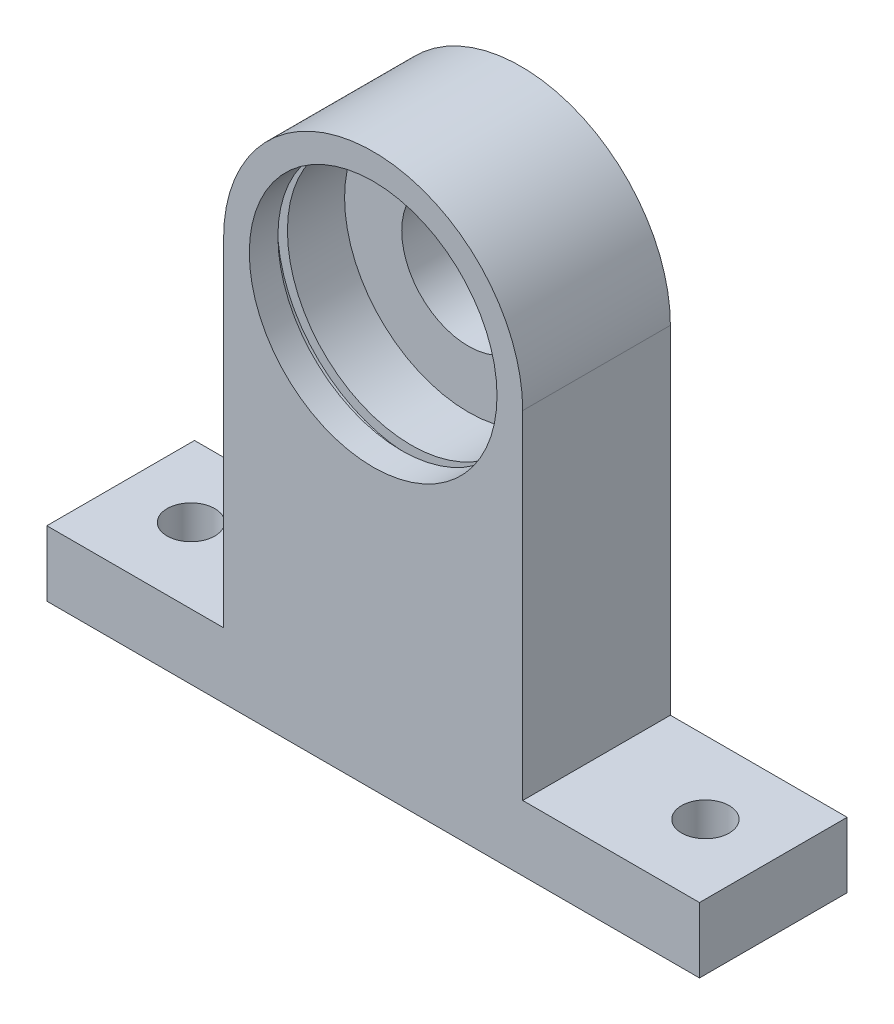
from build123d import *

# Parameters (mm, degrees)
SKETCH1_R           = 31.396947085
SKETCH1_R_2         = 12.5
BOSS_EXTRUDE1_DEPTH = 31
SKETCH2_R           = 5
CUT_EXTRUDE1_DEPTH  = 31
SKETCH3_R           = 14
CUT_EXTRUDE2_DEPTH  = 114.19357359
SKETCH5_R           = 26
CUT_EXTRUDE4_DEPTH  = 20
SKETCH6_R           = 28.1
CUT_EXTRUDE5_DEPTH  = 2


with BuildPart() as part:
    # Sketch1 → Boss-Extrude1 (new body)
    # profile 1 of 2: a face of its own
    with BuildSketch(Plane.XY):
        Circle(SKETCH1_R)
        with Locations(Location((0, 0, 0), (0, 0, 180))):
            Circle(SKETCH1_R_2, mode=Mode.SUBTRACT)
    # profile 2 of 2: a face of its own
    with BuildSketch(Plane.XY):
        with BuildLine():
            ThreePointArc((31.396947085, 0), (0, -31.396947085), (-31.396947085, 0))
            Line((-31.396947085, 0), (-31.396947085, -70.888581066))
            Line((-31.396947085, -70.888581066), (-68.506708087, -70.888581066))
            Line((-68.506708087, -70.888581066), (-68.506708087, -84.608605054))
            Line((-68.506708087, -84.608605054), (68.506708087, -84.608605054))
            Line((68.506708087, -84.608605054), (68.506708087, -70.888581066))
            Line((68.506708087, -70.888581066), (31.396947085, -70.888581066))
            Line((31.396947085, -70.888581066), (31.396947085, 0))
        make_face()
    extrude(amount=BOSS_EXTRUDE1_DEPTH)

    # Sketch2 → Cut-Extrude1 (cut)
    with BuildSketch(Plane(origin=(0, -70.888581066, 0), x_dir=(1, 0, 0), z_dir=(0, 1, 0))):
        with Locations(Location((54, -15.251041139, 0), (0, 0, 270))):
            Circle(SKETCH2_R)
        with Locations(Location((-54, -15.251041139, 0), (0, 0, 270))):
            Circle(SKETCH2_R)
    extrude(amount=-CUT_EXTRUDE1_DEPTH, mode=Mode.SUBTRACT)

    # Sketch3 → Cut-Extrude2 (cut, through all)
    with BuildSketch(Plane(origin=(0, 0, 0), x_dir=(-1, 0, 0), z_dir=(0, 0, -1))):
        Circle(SKETCH3_R)
    extrude(amount=-CUT_EXTRUDE2_DEPTH, mode=Mode.SUBTRACT)

    # Sketch5 → Cut-Extrude4 (cut)
    with BuildSketch(Plane.XY.offset(31)):
        Circle(SKETCH5_R)
    extrude(amount=-CUT_EXTRUDE4_DEPTH, mode=Mode.SUBTRACT)

    # Sketch6 → Cut-Extrude5 (cut)
    with BuildSketch(Plane.XY.offset(23)):
        Circle(SKETCH6_R)
    extrude(amount=CUT_EXTRUDE5_DEPTH, mode=Mode.SUBTRACT)


solid = part.part
